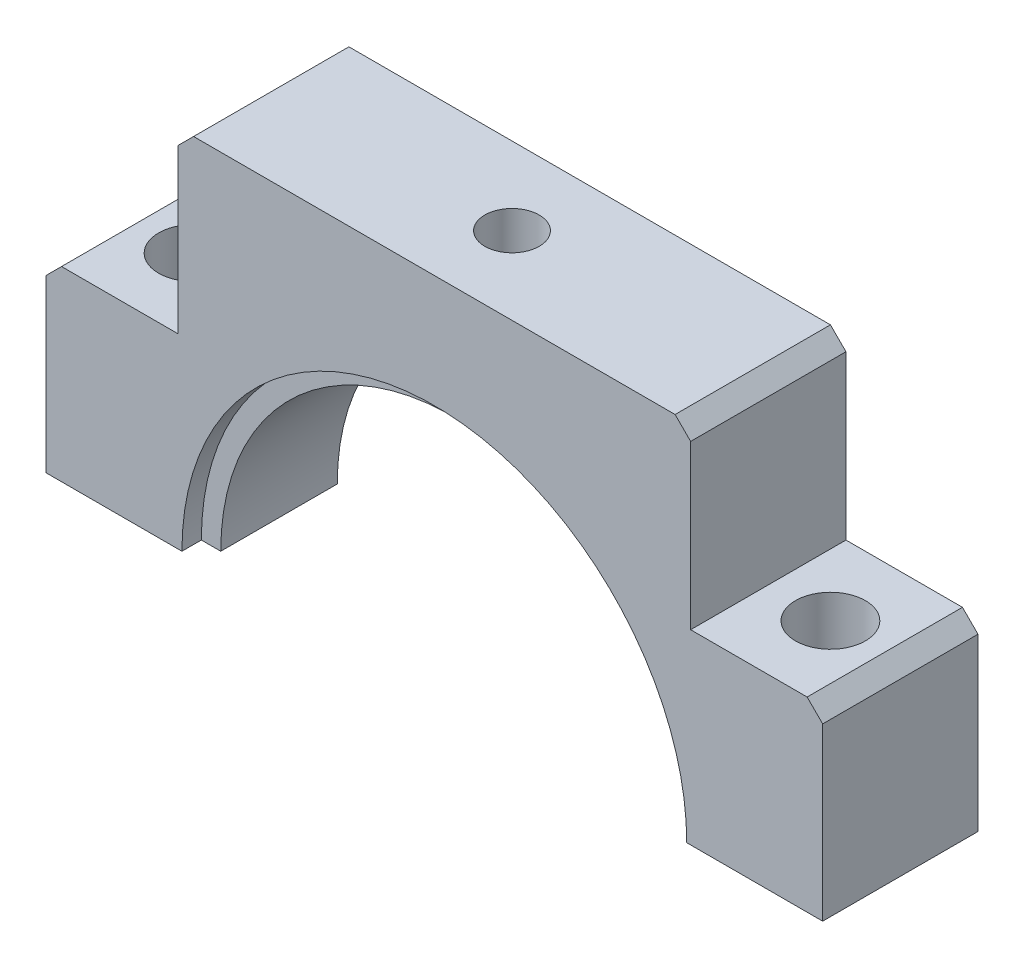
SolidWorks part; units mm, degrees
material "Q235-A"
ref_plane "Front Plane" through (0, 0, 0) normal (0, 0, 1) x (1, 0, 0)
ref_plane "Top Plane" through (0, 0, 0) normal (0, 1, 0) x (1, 0, 0)
ref_plane "Right Plane" through (0, 0, 0) normal (1, 0, 0) x (0, 0, -1)
sketch "Sketch1" plane through (0, 0, 0) normal (0, 0, 1) x (1, 0, 0)
  line L0 (-50, 24) -> (-33, 24)
  line L1 (-50, 0) -> (-30, 0)
  line L2 (-50, 0) -> (-50, 24)
  line L3 (-33, 47) -> (33, 47)
  line L5 (-33, 24) -> (-33, 47)
  line L6 (0, 58.7143) -> (0, -17.0907) construction
  line L7 (50, 0) -> (50, 24)
  line L8 (50, 24) -> (33, 24)
  line L9 (33, 24) -> (33, 47)
  line L10 (30, 0) -> (50, 0)
  arc A0 (30, 0) -> (-30, 0) centre (0, 0) ccw
  point P13 (0, 47)
  dimension "D1" = 100
  dimension "D2" = 47
  dimension "D3" = 23
  dimension "D4" = 33
extrude "Boss-Extrude1" add sketch "Sketch1" along normal blind 20
chamfer "Chamfer1" distance 2 angle 45 4 edges at (50, 24, 10) (33, 47, 10) (-33, 47, 10) (-50, 24, 10)
sketch "Sketch2" plane through (0, 47, 0) normal (0, 1, 0) x (1, 0, 0)
  line L0 (50, -10) -> (-50, -10)
  line L2 (50, 0) -> (50, -20) construction
  line L3 (-50, -20) -> (-50, 0) construction
  line L4 (-41, -1.0808) -> (-41, -18.9192)
  line L5 (41, -1.0808) -> (41, -18.9192)
  point P10 (-41, -10)
  point P11 (41, -10)
  dimension "D1" = 100
  dimension "D2" = 82
  dimension "D3" = 9
hole_wizard "M8x1.0 Tapped Hole1" positions "Sketch3" profile "Sketch4" tap size "M8x1.0" standard "GB"
sketch "Sketch3" plane through (0, 47, 0) normal (0, 1, 0) x (1, 0, 0)
  line L0 (50, -10) -> (-50, -10) construction
  point P0 (0, -10)
sketch "Sketch4" plane through (0, 47, 10) normal (1, 0, 0) x (0, 0, 1)
  line L0 (0, 0) -> (0, 15.103)
  line L1 (0, 15.103) -> (3.5, 13)
  line L2 (3.5, 13) -> (3.5, 0)
  line L5 (3.5, 0) -> (0, 0)
  line L10 (0, 15.103) -> (-3.5, 13) construction
  line L11 (0, -6.35) -> (0, 107.95) construction
  dimension "螺纹孔钻头直径" = 7
  dimension "螺纹孔钻头深度" = 13
  dimension "导头角度" = 118
cosmetic thread "Cosmetic Thread1" parameters "D1"=8, "D2"=8
hole_wizard "Hole2" positions "Sketch9" profile "Sketch10" legacy end condition through all
sketch "Sketch9" plane through (0, 24, 0) normal (0, 1, 0) x (1, 0, 0)
  line L0 (-41, -1.0808) -> (-41, -18.9192) construction
  line L1 (41, -1.0808) -> (41, -18.9192) construction
  point P0 (-41, -10)
  point P4 (41, -10)
sketch "Sketch10" plane through (-41, 24, 10) normal (1, 0, 0) x (0, 0, 1)
  line L0 (0, 0) -> (0, 24)
  line L1 (0, 24) -> (4.5, 24)
  line L2 (4.5, 24) -> (4.5, 0)
  line L3 (4.5, 0) -> (0, 0)
  line L4 (0, 110) -> (0, -10) construction
  dimension "直径" = 9
  dimension "深度" = 24
sketch "Sketch15" plane through (0, 0, 0) normal (0, 0, -1) x (-1, 0, 0)
  circle A0 centre (0, 0) radius 32.5
extrude "Cut-Extrude3" cut sketch "Sketch15" against normal blind 2.5
sketch "Sketch16" plane through (0, 0, 20) normal (0, 0, 1) x (1, 0, 0)
  circle A1 centre (0, 0) radius 32.5
  circle A2 centre (0, 0) radius 32.5
  dimension "D1" = 0
extrude "Cut-Extrude4" cut sketch "Sketch16" against normal blind 2.5
hole_wizard "Hole3" positions "Sketch18" profile "Sketch19" legacy end condition through all
sketch "Sketch18" plane through (0, 47, 0) normal (0, 1, 0) x (1, 0, 0)
  point P0 (0, -10)
sketch "Sketch19" plane through (0, 47, 10) normal (1, 0, 0) x (0, 0, 1)
  line L0 (0, 0) -> (0, 47)
  line L1 (0, 47) -> (2, 47)
  line L2 (2, 47) -> (2, 0)
  line L3 (2, 0) -> (0, 0)
  line L4 (0, 110) -> (0, -10) construction
  dimension "直径" = 4
  dimension "深度" = 47
